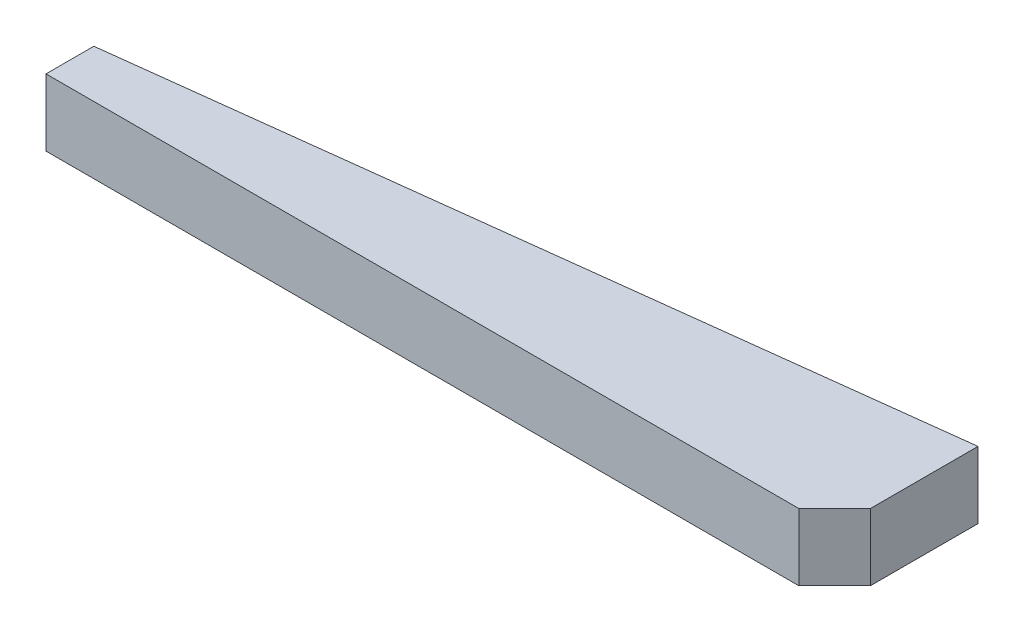
SolidWorks part; units mm, degrees
ref_plane "Front Plane" through (0, 0, 0) normal (0, 0, 1) x (1, 0, 0)
ref_plane "Top Plane" through (0, 0, 0) normal (0, 1, 0) x (1, 0, 0)
ref_plane "Right Plane" through (0, 0, 0) normal (1, 0, 0) x (0, 0, -1)
sketch "Sketch1" plane through (0, 0, 0) normal (0, 1, 0) x (1, 0, 0)
  line L0 (2750.8726, 1604.1628) -> (3065.8726, 1604.1628)
  line L1 (3065.8726, 1604.1628) -> (3080.8726, 1619.1628)
  line L2 (3080.8726, 1619.1628) -> (3080.8726, 1664.1628)
  line L3 (3080.8726, 1664.1628) -> (2750.8726, 1624.1628)
  line L4 (2750.8726, 1624.1628) -> (2750.8726, 1604.1628)
extrude "Boss-Extrude1" add sketch "Sketch1" along normal blind 28
